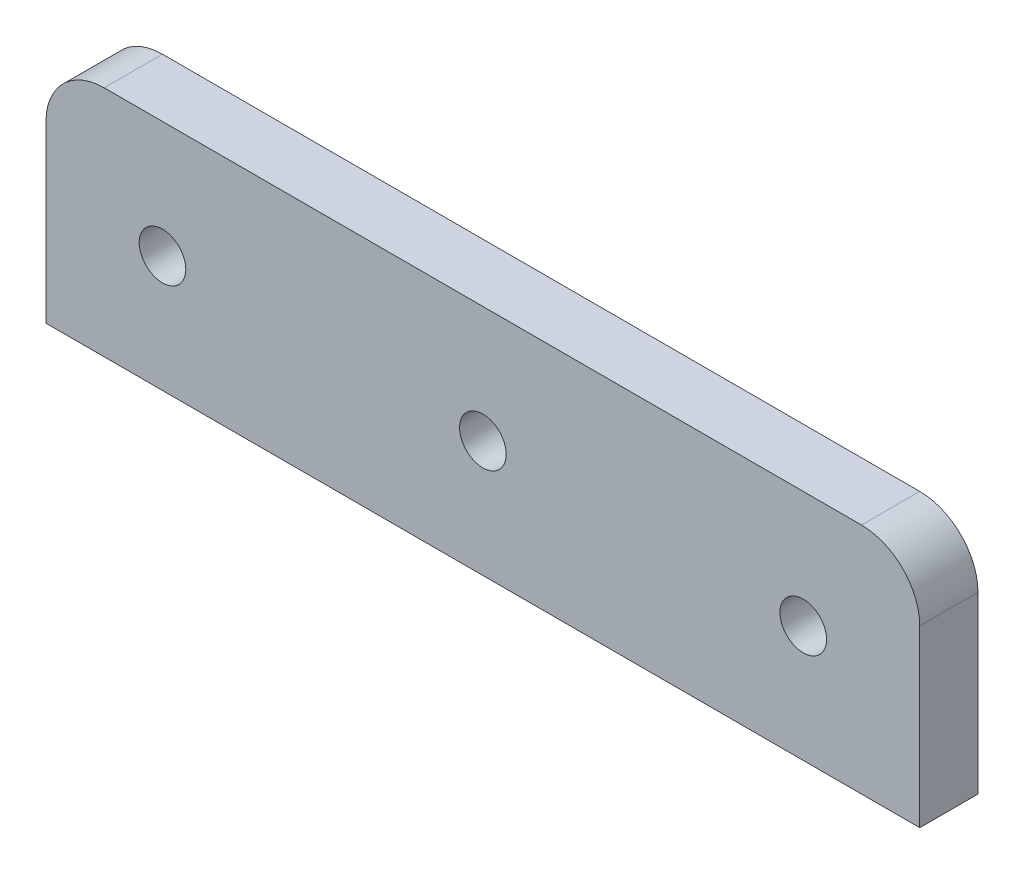
from build123d import *

# Parameters (mm, degrees)
SKETCH1_W           = 75
SKETCH1_H           = 20
SKETCH1_R           = 2
BOSS_EXTRUDE1_DEPTH = 5
FILLET1_R           = 5


with BuildPart() as part:
    # Sketch1 → Boss-Extrude1 (new body)
    with BuildSketch(Plane.XY):
        with Locations((37.5, -10)):
            Rectangle(SKETCH1_W, SKETCH1_H)
        with Locations((10, -10)):
            Circle(SKETCH1_R, mode=Mode.SUBTRACT)
        with Locations((65, -10)):
            Circle(SKETCH1_R, mode=Mode.SUBTRACT)
        with Locations((37.5, -10)):
            Circle(SKETCH1_R, mode=Mode.SUBTRACT)
    extrude(amount=BOSS_EXTRUDE1_DEPTH)

    # Fillet1
    fillet1_edges = [part.edges().sort_by_distance(p)[0] for p in [
        (0, 0, 2.5),
        (75, 0, 2.5),
    ]]
    fillet(fillet1_edges, radius=FILLET1_R)


solid = part.part
